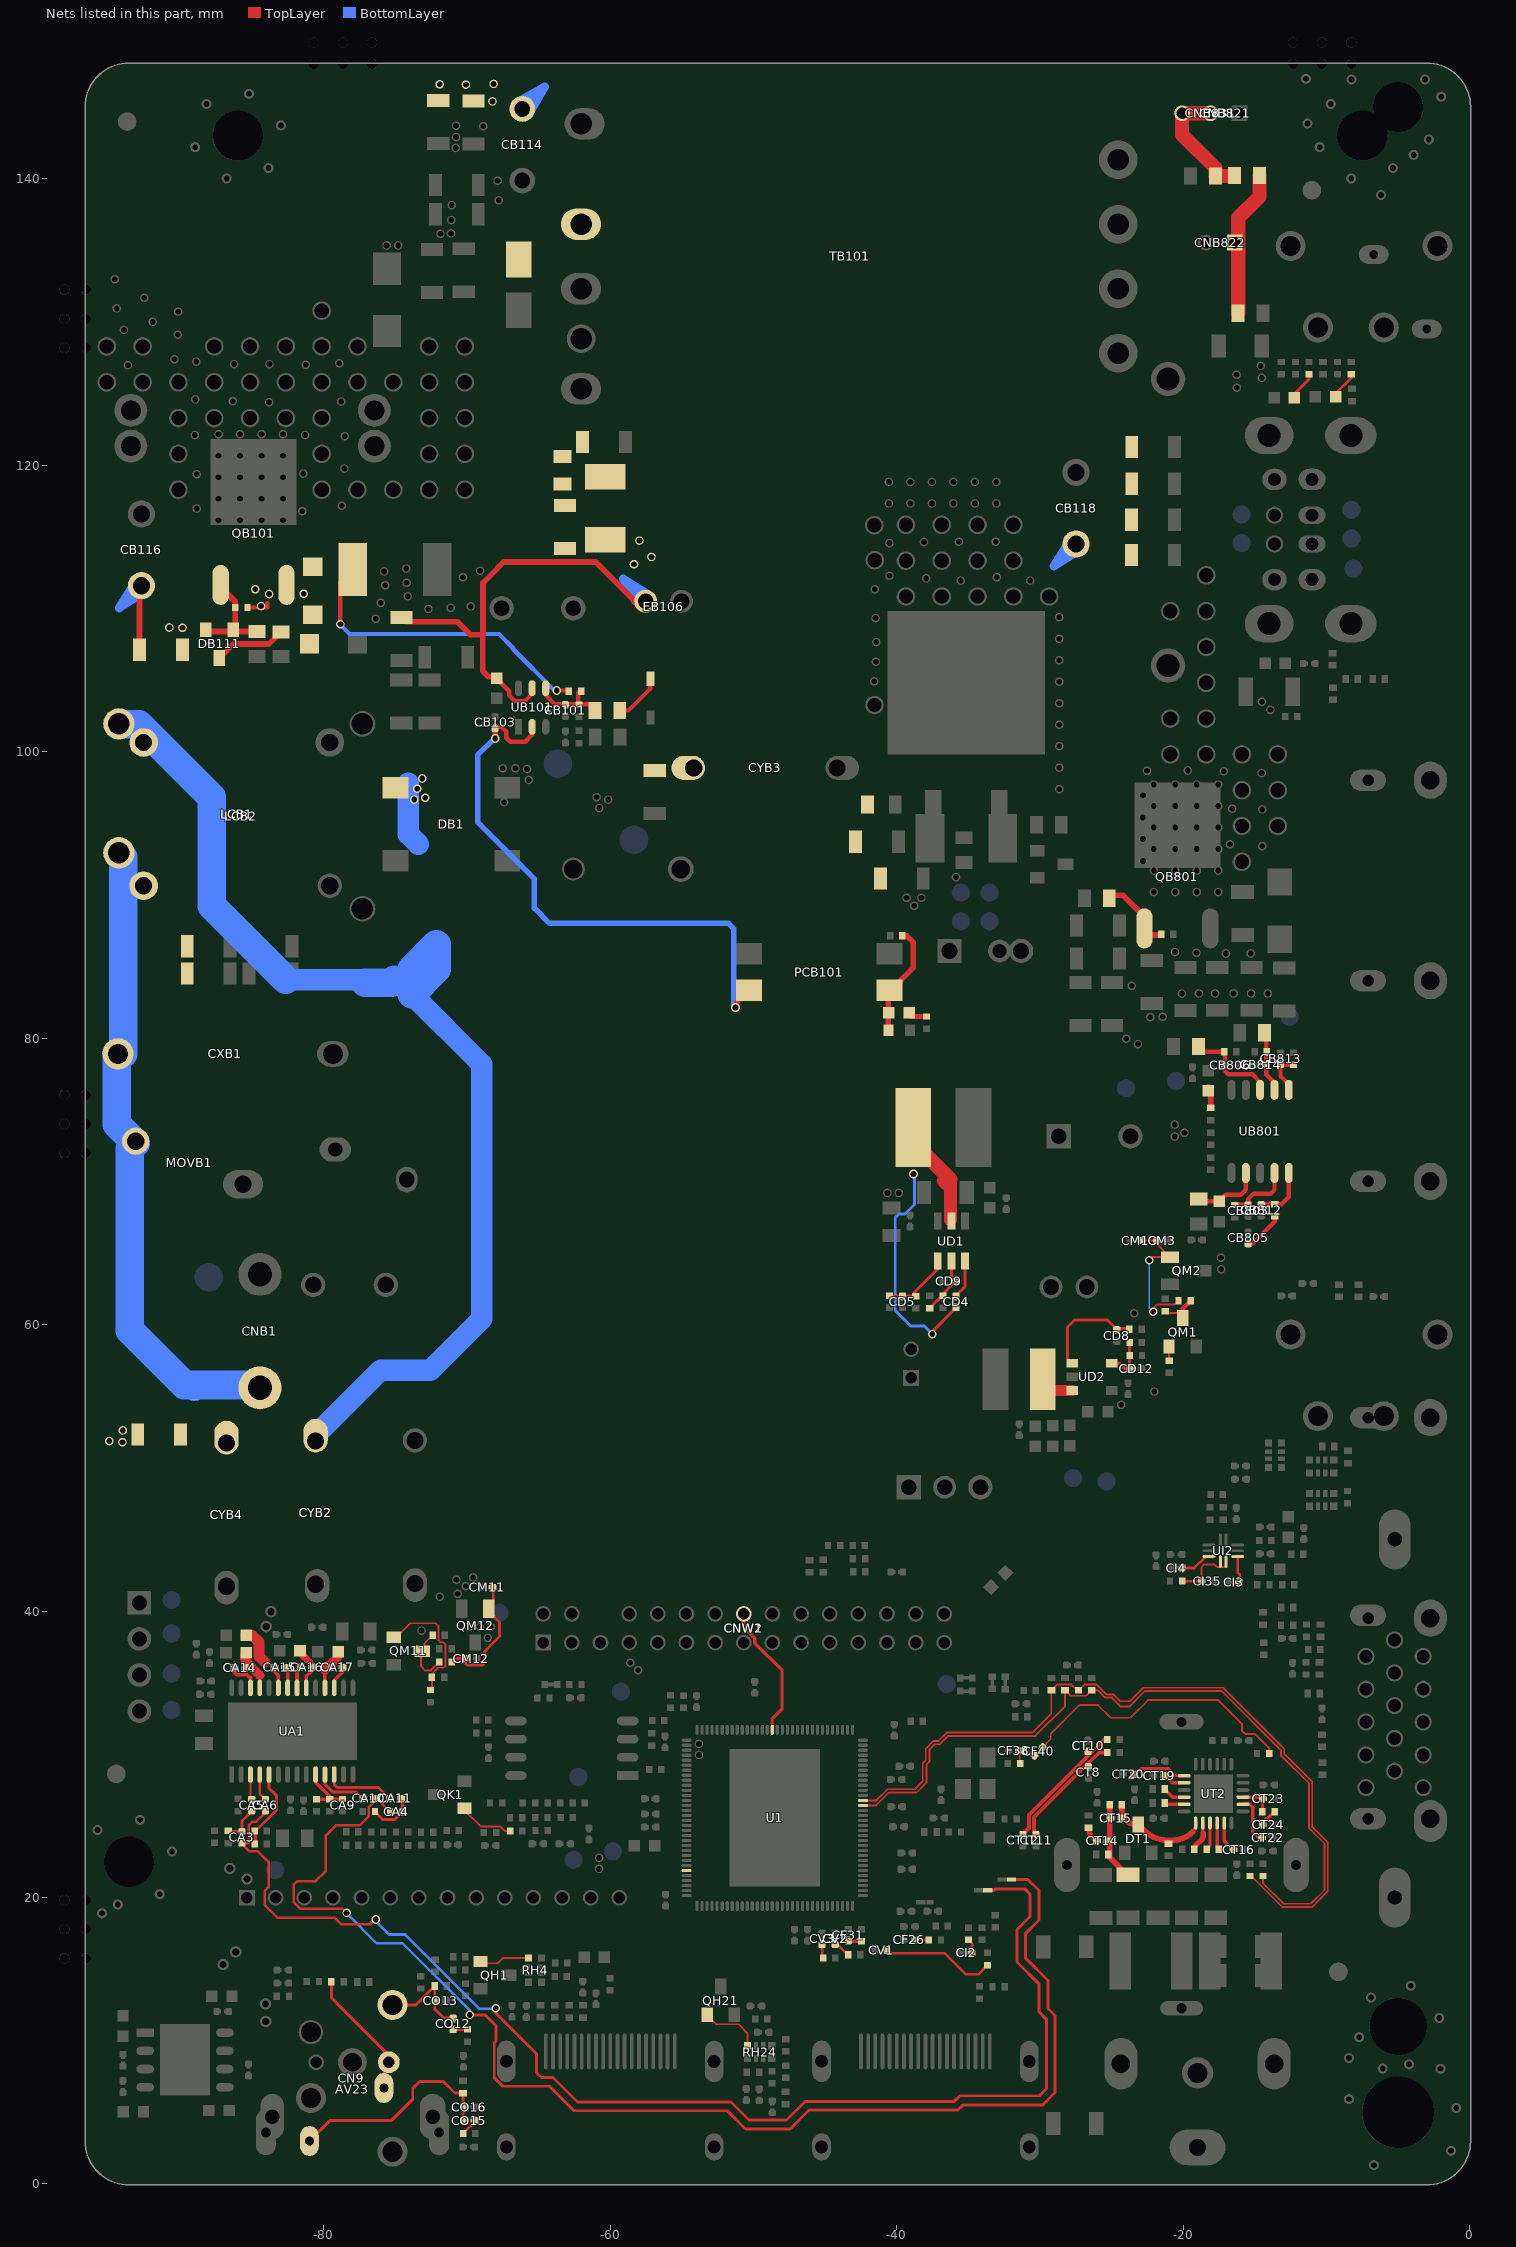
[diagram p0: the nets of this part, all layers, seen from the top]
# Altium PCB MISC86372.PcbDoc (part 12 of 16)
Units mm, origin at the board's own origin, x right, y up, seen from the top; angles counter-clockwise.
Board outline 96.73 x 148.13 mm, 2 copper layers (TopLayer, BottomLayer), stack 1.571 mm thick; 578 components, 318 nets, 2702 pads, 836 vias.

## Via types
v1: diameter 0.6, hole 0.4, TopLayer to BottomLayer, tented both sides, 816 vias
v2: diameter 0.7, hole 0.5, TopLayer to BottomLayer, tented both sides, 15 vias
v3: diameter 0.8, hole 0.5, TopLayer to BottomLayer, tented both sides, 5 vias

## Nets (pads, with @x,y where several pads share a name; then routed paths per layer and width w, separated by ;. In a path a pad name is that pad's centre, name@x,y a point inside that pad or via, vN(x,y) a via of type N, cw(c..) or ccw(c..) an arc to the next point about the centre after c; other vN are vias at no path point) (continued)
LVDS_OCKP_IC: CNW1.16 CNW2.16 U1.81 | length 9.5
  TopLayer w0.178: -48.7,32.474 -48.7,31.717 U1.81@-48.688,31.707
  TopLayer w0.229: CNW2.16@-50.682,39.796 -50.682,38.879 -49.916,38.114 -49.916,37.765 -48.006,35.855 -48.006,33.168 -48.7,32.474
MAIN_SCL_OUT_IC: DK3.K RF43.2 RT2.1 U1.52 | length 55.9
  TopLayer w0.127: U1.52@-42.362,26.781 -41.424,26.781 -40.646,27.559 -38.739,27.559 -38.184,28.114 -38.184,29.366 -37.972,29.578 -37.972,30.393 -37.436,30.928 -37.088,30.928 -36.503,31.513 -30.538,31.513 -29.21,32.841 DK3.K@-29.21,34.475 -28.82,34.865 -27.805,34.865 -27.415,34.475 RF43.2@-27.305,34.475 -26.915,34.865 -26.048,34.865 -25.364,34.181 -24.881,34.181 -24.399,33.698 -23.731,33.698 -22.784,34.646 -17.219,34.646 -12.954,30.38 -12.954,30.03 -10.99,28.066 -10.99,24.942 -9.911,23.862 -9.911,20.431 -11.003,19.339 -13.091,19.339 -15.251,21.499 RT2.1@-15.345,21.499
MAIN_SDA_IO_IC: DK2.K RF44.2 RT3.1 U1.51 | length 54.8
  TopLayer w0.127: U1.51@-42.362,26.431 -41.451,26.431 -40.551,27.33 -38.608,27.33 -37.93,28.009 -37.93,29.261 -37.718,29.473 -37.718,30.324 -37.341,30.7 -36.993,30.7 -36.409,31.284 -30.323,31.284 -28.245,33.362 DK2.K@-28.245,34.475 ; -28.245,33.87 DK2.K@-28.245,34.475 ; RT3.1@-14.43,21.499 -14.43,21.002 -12.996,19.568 -11.097,19.568 -10.139,20.526 -10.139,23.768 -11.219,24.847 -11.219,27.971 -13.183,29.935 -13.183,30.286 -17.314,34.417 -22.689,34.417 -23.781,33.325 -24.349,33.325 -24.976,33.952 -25.459,33.952 -25.981,34.475 RF44.2@-26.391,34.475 -26.781,34.084 -27.855,34.084 DK2.K@-28.245,34.475
MHL_5V_IN_IC: U1.123
MINIAV_LOUT: CN9.3 CO12.1 CO13.2@-72.081,12.802 CO13.2@-72.256,12.802 DI6.K | length 6.6
  TopLayer w0.203: CN9.3@-75.2,12.5 -73.577,12.5 -72.259,13.818 DI6.K@-72.256,13.818 CO13.2@-72.256,12.802 -72.256,12.211 -71.646,11.601 CO12.1@-70.968,11.601
MINIAV_LOUT&OPT: AV23.3 CN9.6 RO4.2 | length 9.3
  TopLayer w0.203: RO4.2@-79.47,14.118 -79.47,12.998 -78.743,12.271 ; -78.813,12.341 -78.743,12.271 ; CN9.6@-75.8,6.7 -75.8,8.16 AV23.3@-75.46,8.5 -75.46,8.988 -78.743,12.271
MINIAV_ROUT: CN9.2 CO15.1 CO16.2@-70.1,5.371 CO16.2@-70.275,5.371 DI8.K | length 15.5
  TopLayer w0.203: CN9.2@-81,3 -79.555,4.445 -75.26,4.445 -73.787,5.918 -73.787,6.68 -73.304,7.163 -71.661,7.163 -70.841,6.343 DI8.K@-70.275,6.343 CO16.2@-70.275,5.131 ; CO16.2@-70.275,5.371 -70.275,4.606 CO15.1@-70.1,4.431
N-1: CNB1.3 CXB1.2 LCB1.1 LCB2.1 MOVB1.2@-93.133,72.798 pad.VIA5@-94.031,52.603 pad.VIA5@-94.056,51.791 pad.VIA5@-94.971,51.867 RB3.2 RB4.2 RB143.1 TP_N.1 | length 45
  BottomLayer w2: CXB1.2@-94.444,78.892 -94.444,73.982 -93.133,72.671 -93.548,72.255 -93.548,59.588 -89.743,55.783 CNB1.3@-84.226,55.783 ; LCB2.1@-94.292,92.905 -94.005,92.618 CXB1.2@-94.005,78.892
N-2: CYB2.1 DB1.3 LCB1.4@-92.578,100.635 LCB2.4 pad.VIA5@-72.923,96.774 pad.VIA5@-73.127,98.12 pad.VIA5@-73.482,97.409 pad.VIA5@-73.685,96.647 | length 83.1
  BottomLayer w1.5: -82.321,84.069 -77.111,84.069 ; CYB2.1@-80.239,52.603 -76.038,56.804 -72.554,56.804 -68.961,60.397 -68.961,78.156 -73.869,83.063 ; -75.062,84.069 -73.869,84.069 -73.869,84.805 ; -74.092,97.79 -74.092,94.234 -73.393,93.535
  BottomLayer w2: LCB2.4@-94.292,101.905 -92.913,101.905 -87.833,96.825 -87.833,89.246 -82.656,84.069 ; -77.111,83.859 -75.274,83.859 -75.064,84.069 ; -73.869,83.063 -72.136,84.796 -72.136,86.538 -73.869,84.805
N-3: CYB4.1 RB143.2
NetBA1_1: BA1.1 CA14.2@-85.427,36.043 CA14.2@-85.602,36.043 UA1.25 | length 2.7
  TopLayer w0.254: UA1.25@-84.472,34.661 -84.472,35.519
  TopLayer w0.635: BA1.1@-85.496,36.913 -85.496,36.544 -84.472,35.519
NetBA2_1: BA2.1 CA15.2@-83.327,36.069 CA15.2@-83.502,36.069 UA1.23 | length 4.2
  TopLayer w0.254: CA15.2@-83.502,36.069 -83.502,35.835 -83.172,35.505 UA1.23@-83.172,34.661
  TopLayer w0.762: BA2.1@-85.446,38.278 -84.971,38.278 -84.525,37.832 -84.525,36.839 -84.121,36.436
NetBA3_1: BA3.1 CA16.2@-80.783,36.086 CA16.2@-80.958,36.086 UA1.20 | length 2.8
  TopLayer w0.254: UA1.20@-81.222,34.661 -81.222,35.44 -80.848,35.814 -80.848,35.977 CA16.2@-80.958,36.086 CA16.2@-80.783,36.086
  TopLayer w0.508: BA3.1@-81.547,37.165 -81.547,36.986 -80.965,36.405
NetBA4_1: BA4.1 CA17.2@-79.313,36.068 CA17.2@-79.488,36.068 UA1.18 | length 2.9
  TopLayer w0.254: UA1.18@-79.922,34.661 -79.922,35.895
  TopLayer w0.635: -79.922,35.895 -78.999,36.818 BA4.1@-78.999,37.16
NetBB101_2: BB101.2 TB101.3
NetCA3_1: CA3.1 CA6.1 RA4.JP_1K | length 89.8
  TopLayer w0.178: CA3.1@-85.714,23.749 -85.185,23.22 -84.6,23.22 -83.858,22.477 -83.858,20.725 -84.112,20.471 -84.112,19.457 -83.248,18.593 -79.24,18.593 -78.77,18.123 -76.721,18.123 v1(-76.378,18.466) ; CA3.1@-85.714,23.772 -85.311,23.772 -85.254,23.829 -85.254,25.014 -84.978,25.29 -84.73,25.29 -84.075,25.945 CA6.1@-84.075,26.023
  TopLayer w0.203: v1(-67.996,12.268) -67.996,11.938 -65.151,9.093 -65.151,7.772 -64.808,7.429 -63.993,7.429 -62.288,5.724 -51.576,5.724 -50.309,4.458 -47.691,4.458 -46.378,5.77 -35.979,5.77 -35.588,6.162 -30.033,6.162 -29.557,6.637 -29.557,11.503 -30.058,12.004 -30.058,13.951 -31.61,15.503 -31.61,17.751 -30.688,18.673 -30.688,20.227 -31.065,20.604 -33.091,20.604 -33.198,20.498 RA4.JP_1K@-33.64,20.498
  BottomLayer w0.178: v1(-76.378,18.466) -76.378,18.346 -75.448,17.417 -74.327,17.417 -70.779,13.868 -69.153,12.243 v1@-67.996,12.243
NetCA3_2: CA3.2@-85.714,24.447 CA3.2@-85.714,24.622 CA5.1 RA3.2 | length 2.9
  TopLayer w0.203: RA3.2@-86.672,24.647 -86.704,24.647 -86.679,24.622 CA3.2@-85.714,24.622 -85.714,25.342 CA5.1@-85.033,26.023 ; CA5.1@-84.982,26.023 CA5.1@-84.982,26.198
NetCA4_1: CA4.1 CA11.1 RA14.2 | length 3.3
  TopLayer w0.203: RA14.2@-76.439,26.007 -76.417,25.984 -75.886,25.454 -75.044,25.454 CA4.1@-74.514,25.984 -74.514,26.866 CA11.1@-74.569,26.921
NetCA4_2: CA4.2@-75.189,25.984 CA4.2@-75.364,25.984 CA10.1 RA5.JP_1K | length 93.6
  TopLayer w0.178: v1(-78.41,18.923) -78.711,19.224 -81.646,19.224 -82.105,19.683 -82.105,20.892 -81.851,21.146 -80.569,21.146 -79.858,21.858 -79.858,24.337 -79.58,24.614 -79.159,25.035 -77.489,25.035 -76.849,25.676 -76.849,26.329 -76.439,26.738 CA10.1@-76.439,26.92 -76.3,26.92 CA4.2@-75.364,25.984 ; CA10.1@-76.614,26.92 CA10.1@-76.595,26.9
  TopLayer w0.203: v1(-69.803,11.804) -68.724,11.804 -67.97,11.051 -67.97,9.982 -68.103,9.849 -68.103,7.412 -67.511,6.82 -64.246,6.82 -62.541,5.115 -51.828,5.115 -50.562,3.848 -47.438,3.848 -46.125,5.161 -35.727,5.161 -35.387,5.501 -29.831,5.501 -28.948,6.384 -28.948,11.756 -29.448,12.256 -29.448,14.203 -31.001,15.756 -31.001,17.498 -30.078,18.421 -30.078,20.48 -30.861,21.262 RA5.JP_1K@-31.99,21.262
  BottomLayer w0.178: v1@-78.41,18.905 -76.312,16.807 -74.508,16.807 -69.803,12.103 v1(-69.803,11.804)
NetCA5_2: CA5.2@-85.033,26.698 CA5.2@-85.033,26.873 UA1.3 | length 1.8
  TopLayer w0.152: UA1.3@-85.122,28.611 -85.122,28.561 -85.122,27.013 CA5.2@-84.982,26.873
NetCA6_2: CA6.2@-84.075,26.698 CA6.2@-84.075,26.873 UA1.4 | length 1.9
  TopLayer w0.152: UA1.4@-84.472,28.561 -84.472,27.227 CA6.2@-84.076,26.831
NetCA9_2: CA9.2@-78.689,26.698 CA9.2@-78.689,26.873 RA10.2 RA11.2 UA1.10 | length 4.1
  TopLayer w0.254: RA10.2@-80.622,26.937 RA10.2@-80.502,26.937 ; UA1.10@-80.572,28.611 -80.572,28.561 -80.572,28.055 RA11.2@-79.454,26.937 ; RA10.2@-80.567,26.848 CA9.2@-78.691,26.848
NetCA10_2: CA10.2@-77.114,26.92 CA10.2@-77.289,26.92 UA1.11 | length 3.7
  TopLayer w0.203: UA1.11@-79.922,28.611 -79.922,28.561 -79.922,27.908 -79.366,27.352 -77.722,27.352 CA10.2@-77.289,26.92
NetCA11_2: CA11.2@-75.244,26.921 CA11.2@-75.419,26.921 UA1.12 | length 5
  TopLayer w0.203: UA1.12@-79.272,28.611 -79.272,27.872 -79.082,27.683 -76.181,27.683 CA11.2@-75.419,26.921
NetCA14_1: CA14.1 UA1.26 | length 2.3
  TopLayer w0.254: CA14.1@-86.277,36.043 -86.277,35.749 -86.088,35.56 -85.362,35.56 -85.122,35.319 UA1.26@-85.122,34.661
NetCA15_1: CA15.1 UA1.22 | length 1.4
  TopLayer w0.254: CA15.1@-82.615,36.068 -82.522,35.975 UA1.22@-82.522,34.661
NetCA16_1: CA16.1 UA1.21 | length 1.5
  TopLayer w0.254: UA1.21@-81.872,34.661 -81.872,35.847 CA16.1@-81.633,36.086
NetCA17_1: CA17.1 UA1.17 | length 1.7
  TopLayer w0.254: UA1.17@-79.272,34.661 -79.272,35.162 -78.994,35.44 -78.686,35.748 -78.638,35.795 CA17.1@-78.638,36.068
NetCA31_1: CA31.1 RA33.1 | length 1.8
  TopLayer w0.203: CA31.1@-12.278,124.943 -11.227,125.994 RA33.1@-11.227,126.346
NetCA32_1: CA32.1 RA34.1 | length 1.8
  TopLayer w0.203: CA32.1@-9.365,124.993 -8.27,126.089 RA34.1@-8.27,126.346
NetCB101_1: CB101.1 RB103.2 RB105.1 RB121.2 UB101.4 | length 5.7
  TopLayer w0.3: UB101.4@-64.506,104.427 -64.506,103.952 -63.849,103.295 CB101.1@-63.129,103.295 RB103.2@-62.214,103.295 ; RB105.1@-62.24,104.14 -62.24,103.321 RB103.2@-62.214,103.295 ; RB103.2@-62.189,103.27 RB103.2@-62.214,103.295 ; RB121.2@-61.074,102.87 -61.499,103.295 RB103.2@-62.214,103.295 ; RB121.2@-60.944,103.101 -61.074,102.972 RB121.2@-60.82,102.972
NetCB102_1: CB102.1 DB104.K EB106.1 pad.VIA5@-57.125,113.589 pad.VIA5@-57.963,114.732 pad.VIA5@-58.344,113.081 RB102.1 RB120.1 UB101.5 | length 30.6
  TopLayer w0.3: CB102.1@-68.067,105.227 -67.056,104.216 -67.056,103.911 -66.668,103.524 -65.945,103.524 -65.456,104.013 UB101.5@-65.456,104.427
  TopLayer w0.4: RB102.1@-74.574,109.348 -74.294,109.068 -70.663,109.068 -69.748,108.153 -68.88,108.153 ; CB102.1@-68.067,105.227 -68.499,105.227 -68.902,105.631 -68.902,108.131 -68.88,108.153 ; EB106.1@-58.268,110.49 -61.011,113.233 -67.462,113.233 -67.847,112.849 -67.847,112.812 -68.88,111.779 -68.88,108.153
  TopLayer w0.6: EB106.1@-58.268,110.49 EB106.1@-57.531,110.49
NetCB103_1: CB103.1 PCB101.4 UB101.2 | length 40.7
  TopLayer w0.3: CB103.1@-68.047,101.712 -67.575,101.712 -67.259,101.397 -67.259,100.965 -66.98,100.686 -65.938,100.686 -65.456,101.168 UB101.2@-65.456,101.727 UB101.2@-65.456,101.85
  TopLayer w0.381: CB103.1@-68.047,101.712 -68.021,101.687 v1(-68.021,100.914) ; v1(-51.256,82.135) -51.256,82.397 PCB101.4@-50.315,83.337 PCB101.4@-50.4,83.337
  BottomLayer w0.381: v1(-68.021,100.914) -68.097,100.914 -69.266,99.746 -69.266,95.072 -65.303,91.11 -65.303,89.078 -64.232,88.007 -51.745,88.007 -51.365,87.627 v1@-51.365,82.135
NetCB109_2: CB109.2 RB133.2 | length 1.2
  TopLayer w0.381: CB109.2@-18.263,76.586 -18.085,76.408 -18.085,75.431
NetCB114_2: CB114.2 pad.VIA5@-68.148,146.609 pad.VIA5@-68.224,145.39 pad.VIA5@-70.079,146.558 pad.VIA5@-71.907,146.583 RB117.2 RB118.2
NetCB116_2: CB116.2 RB119.2 | length 4.5
  TopLayer w0.4: RB119.2@-92.864,107.112 -92.864,111.454 CB116.2@-92.735,111.582
NetCB117_2: CB117.2 RB128.1 RB129.1
NetCB118_2: CB118.2 RB124.2 RB125.2 RB126.2 RB136.2 | length 0.3
  TopLayer w0.6: CB118.2@-27.483,114.188 CB118.2@-27.483,114.492
NetCB119_1: CB119.1 RB120.2
NetCB119_2: CB119.2 DB104.A RB114.1
NetCB139_1: CB139.1 RB139.2 | length 1.3
  TopLayer w0.381: CB139.1@-39.192,81.684 -39.013,81.506 RB139.2@-37.922,81.506
NetCB139_2: CB139.2 PCB101.1 RB131.1 RB132.2 | length 8.1
  TopLayer w0.381: PCB101.1@-40.742,83.111 PCB101.1@-40.589,83.263 ; RB131.1@-40.634,80.442 -40.605,80.471 CB139.2@-40.605,81.684 ; CB139.2@-40.589,81.753 PCB101.1@-40.589,83.263 ; RB132.2@-39.605,87.147 -39.307,87.147 -38.835,86.676 -38.835,84.914 -40.411,83.337 PCB101.1@-40.515,83.337 PCB101.1@-40.589,83.263
NetCB801_1: CB801.1 RB816.2 UB801.2 | length 4.9
  TopLayer w0.3: RB816.2@-19.025,68.608 CB801.1@-17.551,68.608 ; CB801.1@-17.551,68.55 CB801.1@-17.551,68.601 ; CB801.1@-17.501,68.601 -17.039,69.063 -15.977,69.063 -15.63,69.409 UB801.2@-15.63,70.582
NetCB803_1: CB803.1 RB806.2 UB801.4 | length 4.6
  TopLayer w0.3: RB806.2@-16.408,68.345 -16.383,68.37 CB803.1@-15.469,68.37 -15.469,68.758 -15.088,69.139 -13.894,69.139 -13.63,69.402 UB801.4@-13.63,70.582
NetCB805_2: CB805.2@-15.469,65.619 CB805.2@-15.469,65.794 RB804.1 | length 2.8
  TopLayer w0.3: CB805.2@-15.469,65.619 -15.181,65.619 -13.614,67.186 RB804.1@-13.614,67.47
NetCB806_1: CB806.1 RB803.2 RB814.2 UB801.8 | length 6.7
  TopLayer w0.3: RB814.2@-18.946,79.4 -18.59,79.045 RB803.2@-17.138,79.045 -17.081,79.045 -17.081,78.109 -17.085,78.105 -17.085,77.689 -16.866,77.47 -15.164,77.47 -14.63,76.937 UB801.8@-14.63,76.382
NetCB812_2: CB812.2@-14.554,68.221 CB812.2@-14.554,68.396 RB804.2 UB801.5 | length 3.8
  TopLayer w0.3: CB812.2@-14.554,68.396 -13.138,68.396 -12.63,68.904 UB801.5@-12.63,70.582
NetCB813_2: CB813.2@-13.208,78.137 CB813.2@-13.208,78.312 RB813.2 UB801.6 | length 3
  TopLayer w0.3: CB813.2@-13.208,78.312 CB813.2@-13.208,78.133 ; UB801.6@-12.63,76.382 -12.63,76.765 -13.208,77.343 CB813.2@-13.208,78.133 ; RB813.2@-12.421,78.137 -12.425,78.133 CB813.2@-13.208,78.133
NetCB814_1: CB814.1 RB833.2 RB834.1 UB801.7 | length 5.3
  TopLayer w0.3: RB834.1@-14.323,80.366 RB834.1@-14.21,80.25 ; RB834.1@-14.231,80.229 RB834.1@-14.21,80.25 ; RB833.2@-14.205,79.041 -14.205,77.451 -13.63,76.876 UB801.7@-13.63,76.382 ; CB814.1@-14.201,78.126 -14.201,80.241 RB834.1@-14.21,80.25 ; RB834.1@-14.145,80.315 RB834.1@-14.21,80.25
NetCD4_1: CD4.1 LD1.1 UD1.2 | length 23.7
  TopLayer w0.203: v1(-37.516,59.334) -37.595,59.414 -37.595,59.433 CD4.1@-35.859,61.17
  TopLayer w0.9: UD1.2@-36.254,67.296 -36.254,70.155
  TopLayer w1.016: LD1.1@-38.879,73.431 -38.879,72.779 -36.254,70.155 ; -36.673,70.039 -36.467,69.833
  BottomLayer w0.203: v1(-38.829,70.51) -38.76,70.442 -38.76,68.374 -39.418,67.716 -39.853,67.716 -40.107,67.462 -40.107,60.978 -39.022,59.893 -38.075,59.893 v1(-37.516,59.334)
NetCD4_2: CD4.2@-35.859,61.845 CD4.2@-35.859,62.02 UD1.6 | length 2.7
  TopLayer w0.203: CD4.2@-35.859,62.02 -35.239,62.64 UD1.6@-35.239,64.431
NetCD5_1: CD5.1 RD3.1 RD5.2 UD1.4 | length 4.9
  TopLayer w0.203: RD5.2@-40.513,62.014 -40.488,61.989 RD3.1@-38.677,61.989 ; RD3.1@-38.76,62.007 -38.76,62.255 -37.139,63.877 UD1.4@-37.139,64.431
NetCD8_2: CD8.2@-24.638,59.483 CD8.2@-24.638,59.658 RD7.1 UD2.1 | length 7.4
  TopLayer w0.203: UD2.1@-27.74,57.293 -28.072,57.625 -28.072,59.837 -27.584,60.325 -25.31,60.325 -24.7,59.715 RD7.1@-23.806,59.715
NetCD9_2: CD9.2@-35.94,63.017 CD9.2@-36.115,63.017 RD1.2 RD6.2 UD1.5 | length 4.2
  TopLayer w0.203: RD6.2@-37.694,61.145 -36.831,62.007 RD1.2@-36.779,62.007 ; RD1.2@-36.927,61.989 -35.94,62.975 CD9.2@-35.94,63.017 ; UD1.5@-36.189,64.431 -36.189,63.429 CD9.2@-35.859,63.099
NetCD12_1: CD12.1 RD8.1 RD9.2 UD2.5 | length 3.3
  TopLayer w0.203: UD2.5@-24.99,57.293 UD2.5@-24.99,57.293 -24.461,57.293 -24.079,56.911 CD12.1@-23.723,56.911 -23.742,56.93 RD8.1@-23.742,58.75 RD8.1@-23.73,58.738
NetCF26_2: CF26.2@-38.691,17.043 CF26.2@-38.866,17.043 RF12.1 | length 1
  TopLayer w0.203: CF26.2@-38.716,17.043 RF12.1@-37.763,17.043
NetCF31_2: CF31.2@-43.383,16.948 CF31.2@-43.383,17.123 RF16.1 | length 0.9
  TopLayer w0.254: CF31.2@-43.383,16.948 RF16.1@-42.469,16.948
NetCF38_2: CF38.2@-31.408,30.251 CF38.2@-31.583,30.251 CF40.2@-30.4,29.9 CF40.2@-30.276,30.024 RF24.1 | length 2
  TopLayer w0.127: RF24.1@-31.414,29.362 -31.408,29.368 CF38.2@-31.408,30.251 -30.861,30.251 CF40.2@-30.459,29.849
NetCF40_1: CF40.1 L6.1 | length 20.7
  TopLayer w0.127: CF40.1@-29.858,30.45 -29.244,31.064 -29.244,31.443 -27.247,33.439 -25.954,33.439 -25.07,32.555 -23.689,32.555 -22.462,33.782 -17.551,33.782 -17.018,33.249 ; -17.365,33.596 -17.018,33.249 ; L6.1@-14.002,30.041 -14.002,30.427 -14.995,31.42 -15.392,31.42 -15.672,31.42 -15.905,31.653 -15.905,32.136 -17.018,33.249
NetCI2_1: CI2.1 RI2.1 | length 1
  TopLayer w0.178: RI2.1@-35,17.053 -34.729,16.782 CI2.1@-34.729,16.129
NetCI3_2: CI3.2@-16.046,41.993 CI3.2@-16.221,41.993 RI5.1 UI2.8 | length 2
  TopLayer w0.178: UI2.8@-16.206,43.808 -16.206,42.697 -16.046,42.538 CI3.2@-16.046,41.993 CI3.2@-16.134,42.08
NetCI4_2: CI4.2@-20.071,42.996 CI4.2@-20.246,42.996 RI6.1 UI2.5 | length 2
  TopLayer w0.178: -19.234,42.996 UI2.5@-18.422,43.808
  TopLayer w0.203: RI6.1@-20.071,42.996 -19.234,42.996
NetCI35_1: CI35.1 RI3.2 UI2.6 UI2.7 | length 4.7
  TopLayer w0.127: CI35.1@-18.724,42.026 -18.724,43.055 -18.523,43.256 -17.831,43.256 -17.64,43.065 -17.006,43.065 UI2.7@-17.006,43.458
  TopLayer w0.178: RI3.2@-20.073,42.088 -18.837,42.088 CI35.1@-18.724,41.975
NetCM1_1: CM1.1 CM3.2@-21.703,65.862 CM3.2@-21.878,65.862 QM2.G RM4.2 | length 10
  TopLayer w0.127: CM1.1@-22.855,65.811 -22.804,65.862 CM3.2@-21.878,65.862 -21.877,65.663 QM2.G@-20.926,64.712 -22.156,64.712 v1(-22.377,64.491) ; v1(-22.098,60.884) -22.098,61.112 -21.809,61.401 -20.593,61.401 RM4.2@-20.331,61.663
  BottomLayer w0.127: v1(-22.377,64.491) -22.377,61.163 v1(-22.098,60.884)
NetCM11_1: CM11.1 CM12.2@-69.944,36.68 CM12.2@-70.119,36.68 QM12.G RM14.2 | length 9.4
  TopLayer w0.203: RM14.2@-71.076,36.452 -70.848,36.68 CM12.2@-70.119,36.68 -70.119,36.337 -70.009,36.227 -68.91,36.227 -68.783,36.354 -68.783,37.16 -68.428,37.516 ; -68.647,37.296 -68.428,37.516 ; QM12.G@-68.569,40.059 -68.17,40.458 CM11.1@-68.17,41.652 ; QM12.G@-68.564,40.065 -67.729,39.23 -67.729,38.214 -68.428,37.516
NetCNB821_2: CNB821.2 CNB831.2 CNB831.3 RB845.2 RB846.1 | length 8.3
  TopLayer w1: CNB831.2@-18.081,144.562 CNB831.3@-20.081,144.562 -20.081,143.062 -17.752,140.733 RB845.2@-17.752,140.183 ; RB845.2@-17.625,140.183 RB846.1@-16.713,140.183
NetCNB822_1: CNB822.1 RB846.2 RB847.2 | length 10.2
  TopLayer w1: RB847.2@-16.175,130.607 -16.152,130.63 -16.152,137.264 -14.679,138.737 RB846.2@-14.679,140.208
NetCO12_2: CO12.2@-70.968,10.751 CO12.2@-70.968,10.926 RO12.1 | length 1
  TopLayer w0.203: CO12.2@-70.968,10.751 -70.93,10.788 RO12.1@-69.977,10.788
NetCO15_2: CO15.2@-69.6,4.431 CO15.2@-69.425,4.431 RO15.1 | length 1.3
  TopLayer w0.203: RO15.1@-70.275,3.516 -69.425,4.367 CO15.2@-69.425,4.431
NetCT8_2: CT8.2@-26.619,28.978 CT8.2@-26.619,29.153 CT11.2@-30.277,24.253 CT11.2@-30.277,24.428 RT4.2 | length 8
  TopLayer w0.254: CT11.2@-30.277,24.428 -30.416,24.568 -30.416,25.609 -26.587,29.439 -26.556,29.439 -25.87,30.124 RT4.2@-25.495,30.124
NetCT10_1: CT10.1 CT12.2@-31.191,24.253 CT12.2@-31.191,24.428 RT5.2 | length 8.9
  TopLayer w0.254: CT12.2@-31.191,24.428 -30.772,24.847 -30.772,25.756 -26.645,29.883 CT10.1@-26.645,30.157 ; CT10.1@-26.423,30.11 RT5.2@-25.495,31.039
NetCT13_2: CT13.2 CT14.1 CT15.1 LT2.1 LT10.2 | length 5.8
  TopLayer w0.401: LT2.1@-25.229,22.888 LT2.1@-25.229,23.012 ; LT10.2@-25.132,26.474 -25.132,23.52 -25.132,22.79 -25.047,22.705 CT13.2@-23.953,21.612 ; CT13.2@-24.038,21.668 ccw(c-23.852,21.854) CT13.2@-23.953,21.612 ; CT13.2@-23.953,21.612 ccw(c-23.852,21.854) CT13.2@-23.852,21.591 -23.933,21.591 CT13.2@-23.953,21.612
NetCT14_2: CT14.2@-25.904,23.952 CT14.2@-26.079,23.952 LT3.1 | length 1.1
  TopLayer w0.381: LT3.1@-26.619,24.873 ccw(c-25.699,24.873) -26.35,24.223 CT14.2@-26.079,23.952
NetCT15_2: CT15.2@-24.281,25.535 CT15.2@-24.456,25.535 DT1.2 LT4.1 LT10.1 UT2.1 | length 7.2
  TopLayer w0.198: UT2.1@-19.132,25.065 UT2.1@-19.132,25.204
  TopLayer w0.249: -19.329,24.587 ccw(c-19.807,25.065) -19.132,25.065 UT2.1@-19.132,25.204
  TopLayer w0.401: LT10.1@-24.282,26.474 -24.282,26.17 ccw(c-23.157,26.17) -23.952,25.375 ccw(c-23.28,26.047) -23.28,25.096 DT1.2@-23.139,25.096 -22.71,24.667 ccw(c-21.107,26.27) -21.107,24.003 -20.74,24.003 ccw(c-20.74,25.998) -19.329,24.587
NetCT16_1: CT16.1 UT2.5 | length 2.1
  TopLayer w0.229: UT2.5@-17.132,25.204 -17.132,23.92 CT16.1@-16.554,23.343
NetCT19_2: CT19.2@-21.266,28.504 CT19.2@-21.441,28.504 UT2.20 | length 1.5
  TopLayer w0.229: CT19.2@-21.266,28.504 -20.767,28.004 UT2.20@-19.932,28.004
NetCT20_1: CT20.1 UT2.19 | length 3.9
  TopLayer w0.203: CT20.1@-23.422,28.554 -23.422,28.524 -22.944,29.002 -21.032,29.002 -20.534,28.504 UT2.19@-19.932,28.504
NetCT22_1: CT22.1 UT2.8 | length 3.3
  TopLayer w0.229: UT2.8@-15.832,26.504 -15.354,26.504 -15.14,26.291 -15.14,24.549 -14.745,24.154 CT22.1@-14.542,24.154
NetCT23_2: CT23.2@-14.3,26.903 CT23.2@-14.475,26.903 RT6.2 UT2.9 | length 2.3
  TopLayer w0.229: UT2.9@-15.832,27.004 CT23.2@-14.5,27.004 ; CT23.2@-14.5,26.877 CT23.2@-14.475,26.903 RT6.2@-14.474,25.988
NetCT24_2: CT24.2@-14.322,25.07 CT24.2@-14.497,25.07 RT6.1 | length 1.4
  TopLayer w0.127: RT6.1@-13.624,25.988 RT6.1@-13.596,25.959
  TopLayer w0.229: CT24.2@-14.497,25.07 -14.497,25.254 -14.254,25.497 -14.141,25.497 RT6.1@-13.624,26.014
NetCV1_1: CV1.1 RV2.2 | length 7.9
  TopLayer w0.184: CV1.1@-40.597,16.307 -40.402,16.112 -36.653,16.112 -35.179,14.637 -34.298,14.637 RV2.2@-33.655,15.28
NetCV2_1: CV2.1 RV4.2 | length 1.2
  TopLayer w0.183: CV2.1@-44.233,16.695 -44.298,16.695 -44.095,16.695 RV4.2@-43.402,16.002
NetCV3_1: CV3.1 RV10.2 | length 1
  TopLayer w0.183: CV3.1@-45.215,16.695 -45.215,15.859 RV10.2@-45.129,15.773
NetCYB3_1: CYB3.1 RB130.2
NetDB107_K: DB107.K RB121.1 | length 3.5
  TopLayer w0.3: RB121.1@-59.342,102.87 -58.724,102.87 -57.201,104.393 DB107.K@-57.201,105.084
NetDB109_A: DB109.A pad.VIA5@-81.407,111.023 pad.VIA5@-83.82,110.998 pad.VIA5@-84.379,110.16 pad.VIA5@-84.785,111.328 pad.VIA5@-89.865,108.636 pad.VIA5@-90.78,108.661 QB101.S RB105.2 RB109.1 RB119.1 RB148.2 | length 23.4
  TopLayer w0.3: RB109.1@-85.325,110.058 -83.947,110.058 -83.947,110.363 ; v1(-78.842,108.89) -78.842,111.84 RB148.2@-78.285,112.397 ; v1(-63.729,104.267) -62.941,104.267 RB105.2@-62.89,104.216
  BottomLayer w0.3: v1(-78.842,108.89) -78.842,108.836 -78.21,108.204 -67.758,108.204 -66.772,107.218 -66.772,107.147 -63.892,104.267 v1(-63.729,104.267)
NetDB109_K: DB109.K DB110.A
NetDB111_1: DB111.1 DB111.3 QB101.G RB106.2 RB109.2 | length 7.3
  TopLayer w0.4: DB111.3@-88.24,108.509 -88.113,108.382 RB106.2@-84.658,108.382 ; QB101.G@-87.339,111.621 -86.175,110.457 RB109.2@-86.175,110.058 -86.175,108.668 DB111.1@-86.335,108.509
NetDB111_2: DB111.2 RB107.2 | length 5.1
  TopLayer w0.4: DB111.2@-87.287,106.527 -86.311,107.503 -83.835,107.503 RB107.2@-82.982,108.356
NetLD2_2: LD2.2 UD2.3 | length 1.4
  TopLayer w0.762: LD2.2@-29.186,55.393 UD2.3@-27.74,55.393
NetLT5_1: LT5.1 UT2.2 | length 2.1
  TopLayer w0.249: UT2.2@-18.632,25.204 -18.632,24.518 ccw(c-18.586,24.518) -18.618,24.486
  TopLayer w0.381: LT5.1@-19.235,23.368 cw(c-18.883,23.368) -19.132,23.616 -18.72,24.028 ccw(c-18.965,24.274) -18.618,24.274 -18.618,24.486
NetLT6_1: LT6.1 UT2.4 | length 1.9
  TopLayer w0.229: UT2.4@-17.632,25.204 -17.632,23.492 LT6.1@-17.507,23.368
NetLT6_2: LT6.2 UT2.3 | length 1.9
  TopLayer w0.229: LT6.2@-18.357,23.368 -18.132,23.594 UT2.3@-18.132,25.204
NetLT8_2: LT8.2 UT2.23 | length 1.4
  TopLayer w0.249: LT8.2@-21.292,26.599 -21.197,26.504 UT2.23@-19.932,26.504
NetLT9_1: LT9.1 UT2.22 | length 1.6
  TopLayer w0.249: LT9.1@-21.292,27.564 -20.732,27.004 UT2.22@-19.932,27.004
NetQB801_G: QB801.G RB807.2 RB808.1 | length 5.3
  TopLayer w0.4: RB807.2@-25.169,89.967 -24.206,89.967 -22.99,88.75 -22.99,87.655 -22.532,87.198 RB808.1@-21.685,87.198
NetQH1_B: QH1.B RH4.1 | length 3.6
  TopLayer w0.127: QH1.B@-69.063,15.532 -68.947,15.416 -67.846,15.416 -67.477,15.785 RH4.1@-65.703,15.785
NetQH21_B: QH21.B RH24.2 | length 4.2
  TopLayer w0.127: QH21.B@-53.251,11.786 -52.611,11.146 -51.042,11.146 -50.43,10.534 RH24.2@-50.43,9.649
NetQK1_B: QK1.B RK15.1 | length 4
  TopLayer w0.127: QK1.B@-70.18,26.226 -70.18,26.098 -69.042,24.959 -67.668,24.959 -67.356,24.648 RK15.1@-66.998,24.648 RK15.1@-66.998,24.698
NetQM1_B: QM1.B RM2.2 | length 1.1
  TopLayer w0.127: QM1.B@-20.993,58.471 -20.984,58.462 RM2.2@-20.984,57.404
NetQM1_C: QM1.C RM3.1 RM4.1 | length 2.7
  TopLayer w0.127: RM3.1@-21.252,60.941 -21.124,60.813 QM1.C@-20.028,60.813
  TopLayer w0.305: QM1.C@-20.028,60.453 -20.028,60.813 -20.028,61.116 RM4.1@-19.481,61.663
NetQM11_B: QM11.B RM11.2 RM12.1 | length 8.8
  TopLayer w0.127: QM11.B@-74.955,38.163 -73.977,39.141 -72.187,39.141 -71.984,38.938 -71.984,37.948 -71.857,37.821 -71.658,37.821 -71.5,37.663 -71.5,36.144 -71.608,36.036 -72.018,36.036 -72.453,35.602 -72.453,35.428 -72.441,35.416 RM12.1@-72.441,34.537
  TopLayer w0.203: QM11.B@-74.955,38.163 QM11.B@-74.955,38.189
NetQM11_C: QM11.C RM13.2 RM14.1 | length 4.1
  TopLayer w0.127: QM11.C@-73.126,37.198 -73.211,37.113 -73.211,36.129 -72.938,35.857 -72.521,35.857 RM14.1@-71.926,36.452 ; QM11.C@-72.973,37.198 -72.973,37.73 RM13.2@-72.4,38.303
NetRA8_2: RA8.2 RA9.2 UA1.5 | length 5.8
  TopLayer w0.203: RA8.2@-84.822,24.638 RA8.2@-84.767,24.638 ; RA9.2@-84.767,23.728 RA8.2@-84.767,24.638 ; RA8.2@-84.735,24.638 RA8.2@-84.764,24.638 ; UA1.5@-83.822,28.611 -83.822,28.561 -83.822,27.629 -83.291,27.098 -83.291,26.11 RA8.2@-84.764,24.638 ; RA8.2@-84.767,24.638 RA8.2@-84.764,24.638